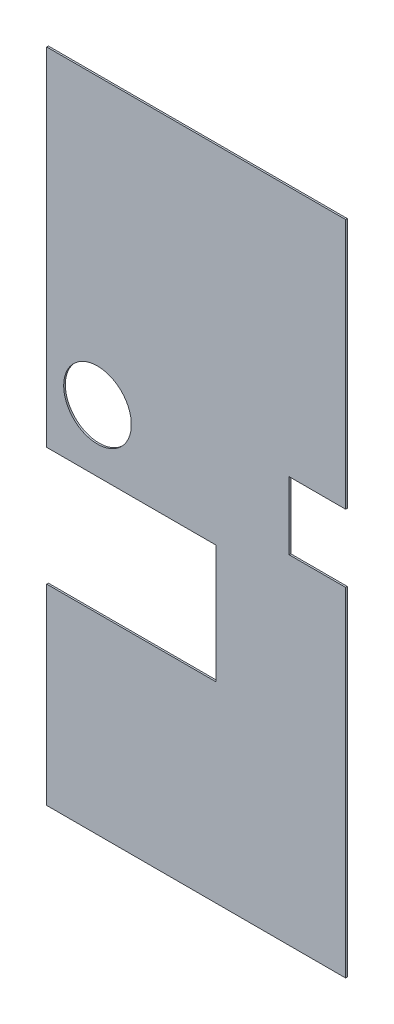
SolidWorks part; units mm, degrees
material "Q235"
ref_plane "Front Plane" through (0, 0, 0) normal (0, 0, 1) x (1, 0, 0)
ref_plane "Top Plane" through (0, 0, 0) normal (0, 1, 0) x (1, 0, 0)
ref_plane "Right Plane" through (0, 0, 0) normal (1, 0, 0) x (0, 0, -1)
sketch "Sketch1" plane through (0, 0, 0) normal (0, 0, 1) x (1, 0, 0)
  line L1 (0, 0) -> (530, 0)
  line L2 (0, 0) -> (0, 340)
  line L3 (0, 340) -> (300, 340)
  line L4 (530, 0) -> (530, 1165)
  line L10 (300, 340) -> (300, 550)
  line L11 (300, 550) -> (0, 550)
  line L12 (0, 550) -> (0, 1165)
  line L13 (0, 1165) -> (530, 1165)
  dimension "D1" = 530
  dimension "D2" = 340
  dimension "D3" = 230
  dimension "D4" = 1165
  dimension "D5" = 210
extrude "Boss-Extrude1" add sketch "Sketch1" along normal blind 3
sketch "Sketch2" plane through (0, 0, 0) normal (0, 0, -1) x (-1, 0, 0)
  line L0 (-490, 660) -> (-90, 660) construction
  line L1 (-430, 600) -> (-550, 600)
  line L2 (-430, 600) -> (-430, 720)
  line L3 (-430, 720) -> (-550, 720)
  line L4 (-550, 600) -> (-550, 720)
  line L5 (-430, 600) -> (-550, 720) construction
  line L6 (-430, 720) -> (-550, 600) construction
  line L7 (-530, 0) -> (-530, 1165) construction
  line L8 (0, 0) -> (-530, 0) construction
  circle A0 centre (-90, 660) radius 60
  point P0 (-490, 660)
  dimension "D3" = 120
  dimension "D1" = 120
  dimension "D2" = 120
  dimension "D4" = 40
  dimension "D5" = 660
  dimension "D6" = 400
extrude "Cut-Extrude1" cut sketch "Sketch2" against normal blind 10
